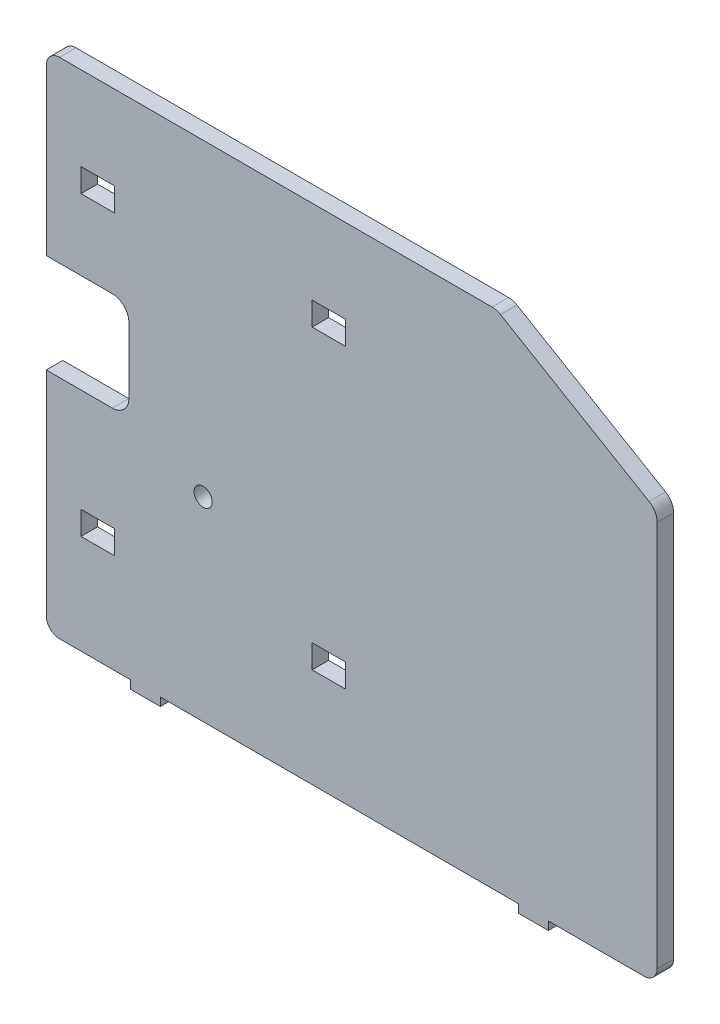
from build123d import *

# Parameters (mm, degrees)
SKETCH1_R           = 5.5
SKETCH1_W           = 20.2
SKETCH1_H           = 14.2
BOSS_EXTRUDE1_DEPTH = 10


with BuildPart() as part:
    # Sketch1 → Boss-Extrude1 (new body)
    with BuildSketch(Plane.XY):
        with BuildLine():
            Line((538.108108788, 869.539360157), (628.108108788, 816.518490855))
            ThreePointArc((628.108108788, 816.518490855), (631.692997782, 812.867012092), (633.002234094, 807.920232682))
            Line((633.002234094, 807.920232682), (633.002234094, 573.941101984))
            ThreePointArc((633.002234094, 573.941101984), (630.659088344, 568.284247734), (625.002234094, 565.941101984))
            Line((625.002234094, 565.941101984), (567.061111031, 565.941101984))
            Line((567.061111031, 565.941101984), (567.061111031, 560.941101984))
            Line((567.061111031, 560.941101984), (549.061111031, 560.941101984))
            Line((549.061111031, 560.941101984), (549.061111031, 565.941101984))
            Line((549.061111031, 565.941101984), (332.061111031, 565.941101984))
            Line((332.061111031, 565.941101984), (332.061111031, 560.941101984))
            Line((332.061111031, 560.941101984), (314.061111031, 560.941101984))
            Line((314.061111031, 560.941101984), (314.061111031, 565.941101984))
            Line((314.061111031, 565.941101984), (271.002234094, 565.941101984))
            ThreePointArc((271.002234094, 565.941101984), (265.345379845, 568.284247734), (263.002234094, 573.941101984))
            Line((263.002234094, 573.941101984), (263.002234094, 702.941101984))
            Line((263.002234094, 702.941101984), (303.002234094, 702.941101984))
            ThreePointArc((303.002234094, 702.941101984), (310.073301906, 705.870034172), (313.002234094, 712.941101984))
            Line((313.002234094, 712.941101984), (313.002234094, 752.941101984))
            ThreePointArc((313.002234094, 752.941101984), (310.073301906, 760.012169796), (303.002234094, 762.941101984))
            Line((303.002234094, 762.941101984), (263.002234094, 762.941101984))
            Line((263.002234094, 762.941101984), (263.002234094, 862.941101984))
            ThreePointArc((263.002234094, 862.941101984), (265.345379845, 868.597956233), (271.002234094, 870.941101984))
            Line((271.002234094, 870.941101984), (533.002234094, 870.941101984))
            ThreePointArc((533.002234094, 870.941101984), (535.649630765, 870.584301187), (538.108108788, 869.539360157))
        make_face()
        with Locations((358.002234094, 683.941101984)):
            Circle(SKETCH1_R, mode=Mode.SUBTRACT)
        with Locations((294.102234094, 633.241101984)):
            Rectangle(SKETCH1_W, SKETCH1_H, mode=Mode.SUBTRACT)
        with Locations((434.102234094, 633.241101984)):
            Rectangle(SKETCH1_W, SKETCH1_H, mode=Mode.SUBTRACT)
        with Locations((294.102234094, 813.041101984)):
            Rectangle(SKETCH1_W, SKETCH1_H, mode=Mode.SUBTRACT)
        with Locations((434.102234094, 813.041101984)):
            Rectangle(SKETCH1_W, SKETCH1_H, mode=Mode.SUBTRACT)
    extrude(amount=BOSS_EXTRUDE1_DEPTH)


solid = part.part
